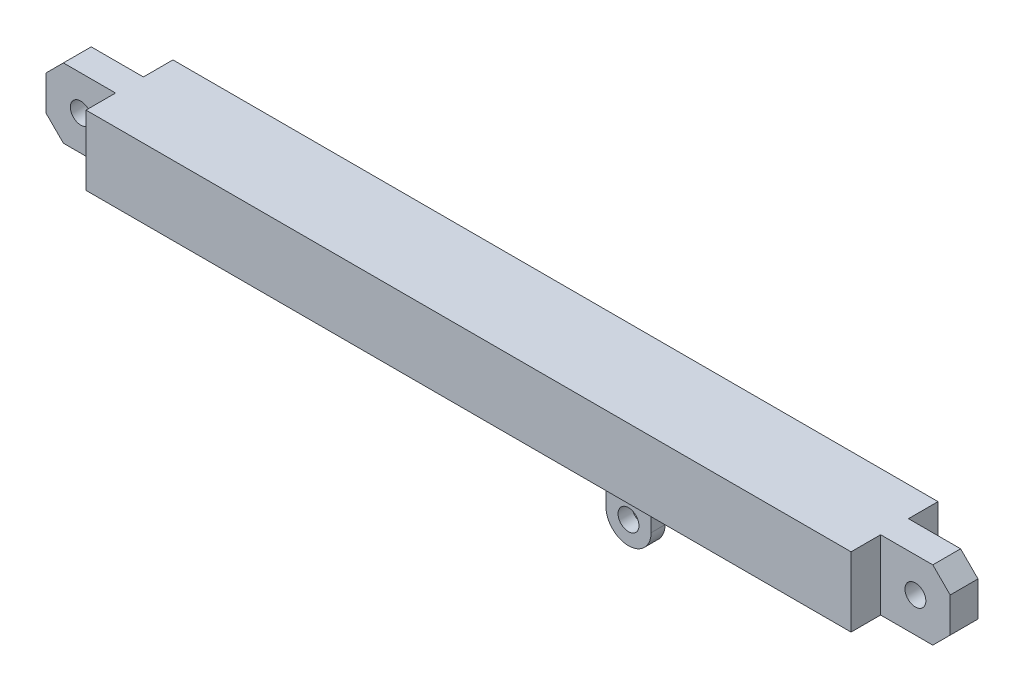
SolidWorks part; units mm, degrees
ref_plane "Front Plane" through (0, 0, 0) normal (0, 0, 1) x (1, 0, 0)
ref_plane "Top Plane" through (0, 0, 0) normal (0, 1, 0) x (1, 0, 0)
ref_plane "Right Plane" through (0, 0, 0) normal (1, 0, 0) x (0, 0, -1)
sketch "Sketch1" plane through (0, 0, 0) normal (0, 0, 1) x (1, 0, 0)
  line L1 (-130, 10) -> (130, 10)
  line L2 (-130, 10) -> (-130, -10)
  line L3 (-130, -10) -> (130, -10)
  line L4 (130, 10) -> (130, -10)
  line L5 (-130, 10) -> (130, -10) construction
  line L6 (-130, -10) -> (130, 10) construction
  point P0 (0, 0)
  dimension "D1" = 260
  dimension "D2" = 20
extrude "Boss-Extrude1" add sketch "Sketch1" along normal mid plane 25
sketch "Sketch2" plane through (0, 0, 12.5) normal (0, 0, 1) x (1, 0, 0)
  line L0 (-130, 10) -> (-130, -10) construction
  line L1 (130, -10) -> (130, 10) construction
  circle A0 centre (-120, 0) radius 3
  circle A1 centre (120, 0) radius 3
  dimension "D2" = 6
  dimension "D1" = 10
  dimension "D3" = 10
extrude "Cut-Extrude1" cut sketch "Sketch2" against normal through all
sketch "Sketch3" plane through (0, 0, 12.5) normal (0, 0, 1) x (1, 0, 0)
  line L0 (-130, 10) -> (-130, -10)
  line L1 (-130, 10) -> (-110, 10)
  line L2 (-130, -10) -> (-110, -10)
  line L3 (-110, 10) -> (-110, -10)
  line L4 (130, 10) -> (130, -10)
  line L5 (130, 10) -> (110, 10)
  line L6 (130, -10) -> (110, -10)
  line L7 (110, 10) -> (110, -10)
  dimension "D1" = 20
  dimension "D2" = 20
extrude "Cut-Extrude2" cut sketch "Sketch3" against normal blind 8.5
mirror "Mirror2" about plane through (0, 0, 0) normal (0, 0, 1) of "Cut-Extrude2"
chamfer "Chamfer1" distance 5 angle 45 4 edges at (130, 10, 0) (130, -10, 0) (-130, -10, 0) (-130, 10, 0)
sketch "Sketch4" plane through (0, 0, -12.5) normal (0, 0, -1) x (-1, 0, 0)
  line L0 (110, -10) -> (-110, -10) construction
  line L1 (-46.5, -20) -> (-46.5, -10)
  line L2 (-46.5, -10) -> (-33.5, -10)
  line L3 (-33.5, -10) -> (-33.5, -20)
  circle A0 centre (-40, -20) radius 3
  arc A1 (-46.5, -20) -> (-33.5, -20) centre (-40, -20) ccw
  dimension "D1" = 6
  dimension "D2" = 13
  dimension "D4" = 40
  dimension "D3" = 10
extrude "Boss-Extrude2" add sketch "Sketch4" against normal blind 4
pattern_linear "LPattern1" count 2 spacing 15 along (0, 0, 1) of "Boss-Extrude2"
